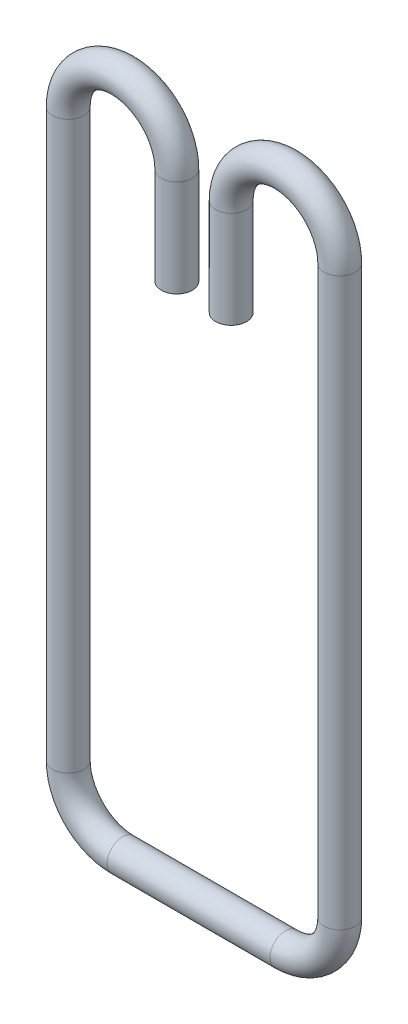
from build123d import *

# Parameters (mm, degrees)
SWEEP_1_PROFILE_R = 8


with BuildPart() as part:
    # 扫描1: sweep along a path in 草图1
    with BuildLine(Plane.XY) as sweep_1_path:
        Line((-14, 270), (-14, 320))
        ThreePointArc((-14, 320), (-42, 348), (-70, 320))
        Line((-70, 320), (-70, 28))
        ThreePointArc((-70, 28), (-61.798989873, 8.201010127), (-42, 0))
        Line((-42, 0), (42, 0))
        ThreePointArc((42, 0), (61.798989873, 8.201010127), (70, 28))
        Line((70, 28), (70, 320))
        ThreePointArc((70, 320), (42, 348), (14, 320))
        Line((14, 320), (14, 270))
    # 扫描1 profile (on start of the path) → 扫描1 (sweep)
    with BuildSketch(Plane(origin=(-14, 270, 0), x_dir=(1, 0, 0), z_dir=(0, 1, 0))):
        Circle(SWEEP_1_PROFILE_R)
    sweep(path=sweep_1_path.line)


solid = part.part
